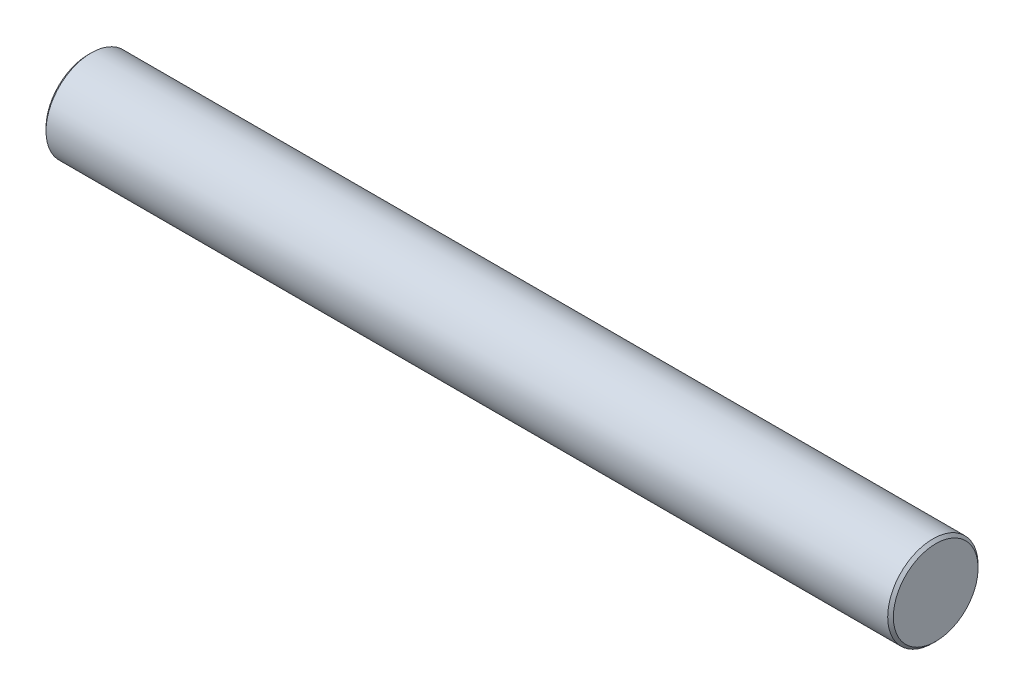
from build123d import *

# Parameters (mm, degrees)
SKETCH_1_W     = 150
SKETCH_1_H     = 8
CHAMFER_1_SIZE = 0.5


with BuildPart() as part:
    # 草图1 → 旋转1 (revolve)
    with BuildSketch(Plane.XY, mode=Mode.PRIVATE) as revolve_1_sk:
        with Locations((0, 4)):
            Rectangle(SKETCH_1_W, SKETCH_1_H)
    revolve(revolve_1_sk.sketch.rotate(Axis((0, 0, 0), (1, 0, 0)), 90), axis=Axis((0, 0, 0), (1, 0, 0)))

    # 倒角1
    chamfer_1_edges = [part.edges().sort_by_distance(p)[0] for p in [
        (-75, 0, -8),
        (75, 0, -8),
    ]]
    chamfer(chamfer_1_edges, length=CHAMFER_1_SIZE)


solid = part.part
